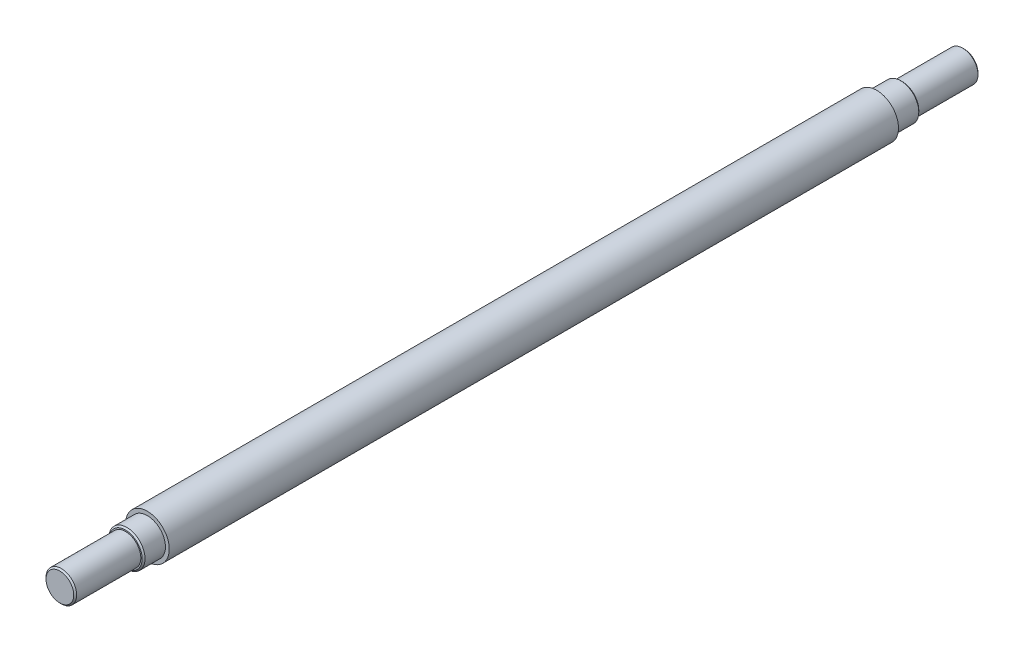
from build123d import *

# Parameters (mm, degrees)
SKETCH1_R           = 21
BOSS_EXTRUDE1_DEPTH = 85
SKETCH2_R           = 24.8
BOSS_EXTRUDE2_DEPTH = 35
SKETCH3_R           = 30
BOSS_EXTRUDE3_DEPTH = 1000
SKETCH4_R           = 24.8
BOSS_EXTRUDE4_DEPTH = 30
SKETCH5_R           = 21
BOSS_EXTRUDE5_DEPTH = 90
CHAMFER2_SIZE       = 2


with BuildPart() as part:
    # Sketch1 → Boss-Extrude1 (new body)
    with BuildSketch(Plane.XY):
        Circle(SKETCH1_R)
    extrude(amount=BOSS_EXTRUDE1_DEPTH)

    # Sketch2 → Boss-Extrude2 (add)
    with BuildSketch(Plane.XY.offset(85)):
        Circle(SKETCH2_R)
    extrude(amount=BOSS_EXTRUDE2_DEPTH)

    # Sketch3 → Boss-Extrude3 (add)
    with BuildSketch(Plane.XY.offset(120)):
        Circle(SKETCH3_R)
    extrude(amount=BOSS_EXTRUDE3_DEPTH)

    # Sketch4 → Boss-Extrude4 (add)
    with BuildSketch(Plane.XY.offset(1120)):
        Circle(SKETCH4_R)
    extrude(amount=BOSS_EXTRUDE4_DEPTH)

    # Sketch5 → Boss-Extrude5 (add)
    with BuildSketch(Plane.XY.offset(1150)):
        Circle(SKETCH5_R)
    extrude(amount=BOSS_EXTRUDE5_DEPTH)

    # Chamfer2
    chamfer2_edges = [part.edges().sort_by_distance(p)[0] for p in [
        (-24.8, 0, 1150),
        (-21, 0, 1240),
        (-21, 0, 0),
        (-24.8, 0, 85),
    ]]
    chamfer(chamfer2_edges, length=CHAMFER2_SIZE)


solid = part.part
